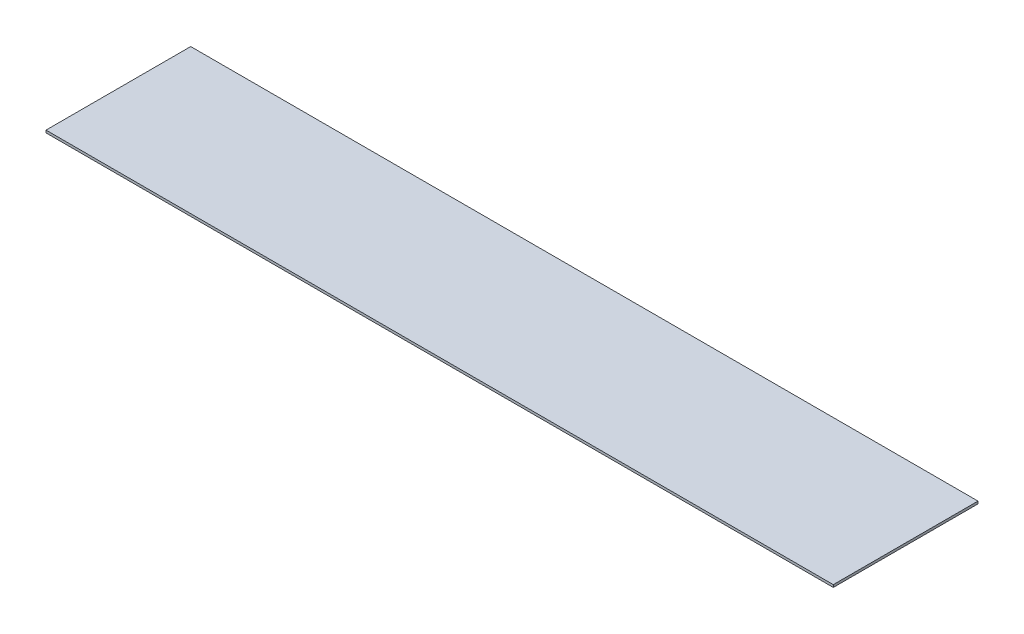
SolidWorks part; units mm, degrees
material "普通碳钢"
ref_plane "Front Plane" through (0, 0, 0) normal (0, 0, 1) x (1, 0, 0)
ref_plane "Top Plane" through (0, 0, 0) normal (0, 1, 0) x (1, 0, 0)
ref_plane "Right Plane" through (0, 0, 0) normal (1, 0, 0) x (0, 0, -1)
sketch "Sketch1" plane through (0, 0, 0) normal (0, 1, 0) x (1, 0, 0)
  line L1 (-321, 59) -> (321, 59)
  line L2 (-321, 59) -> (-321, -59)
  line L3 (-321, -59) -> (321, -59)
  line L4 (321, 59) -> (321, -59)
  line L5 (-321, 59) -> (321, -59) construction
  line L6 (-321, -59) -> (321, 59) construction
  point P0 (0, 0)
  dimension "D1" = 642
  dimension "D2" = 118
extrude "Boss-Extrude1" add sketch "Sketch1" along normal blind 2
